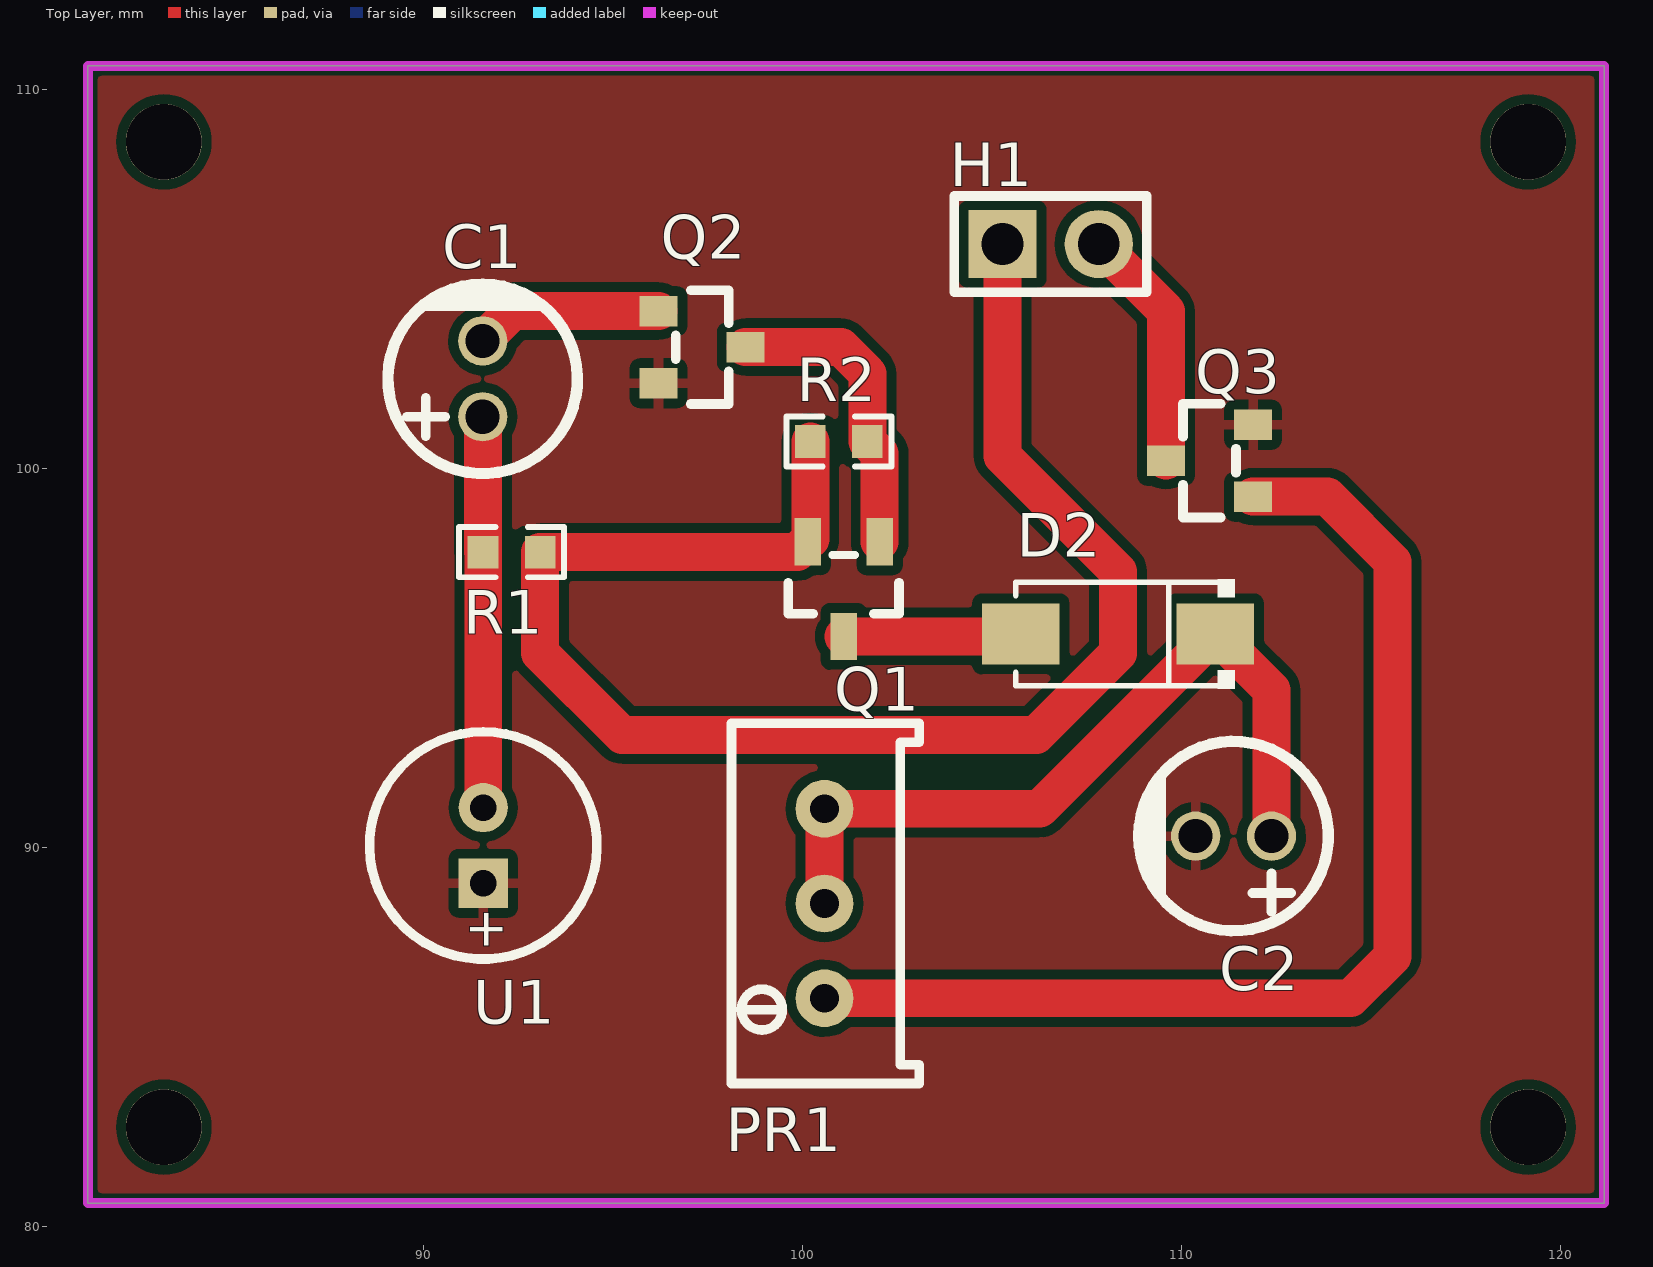
[diagram p0: Top Layer view]
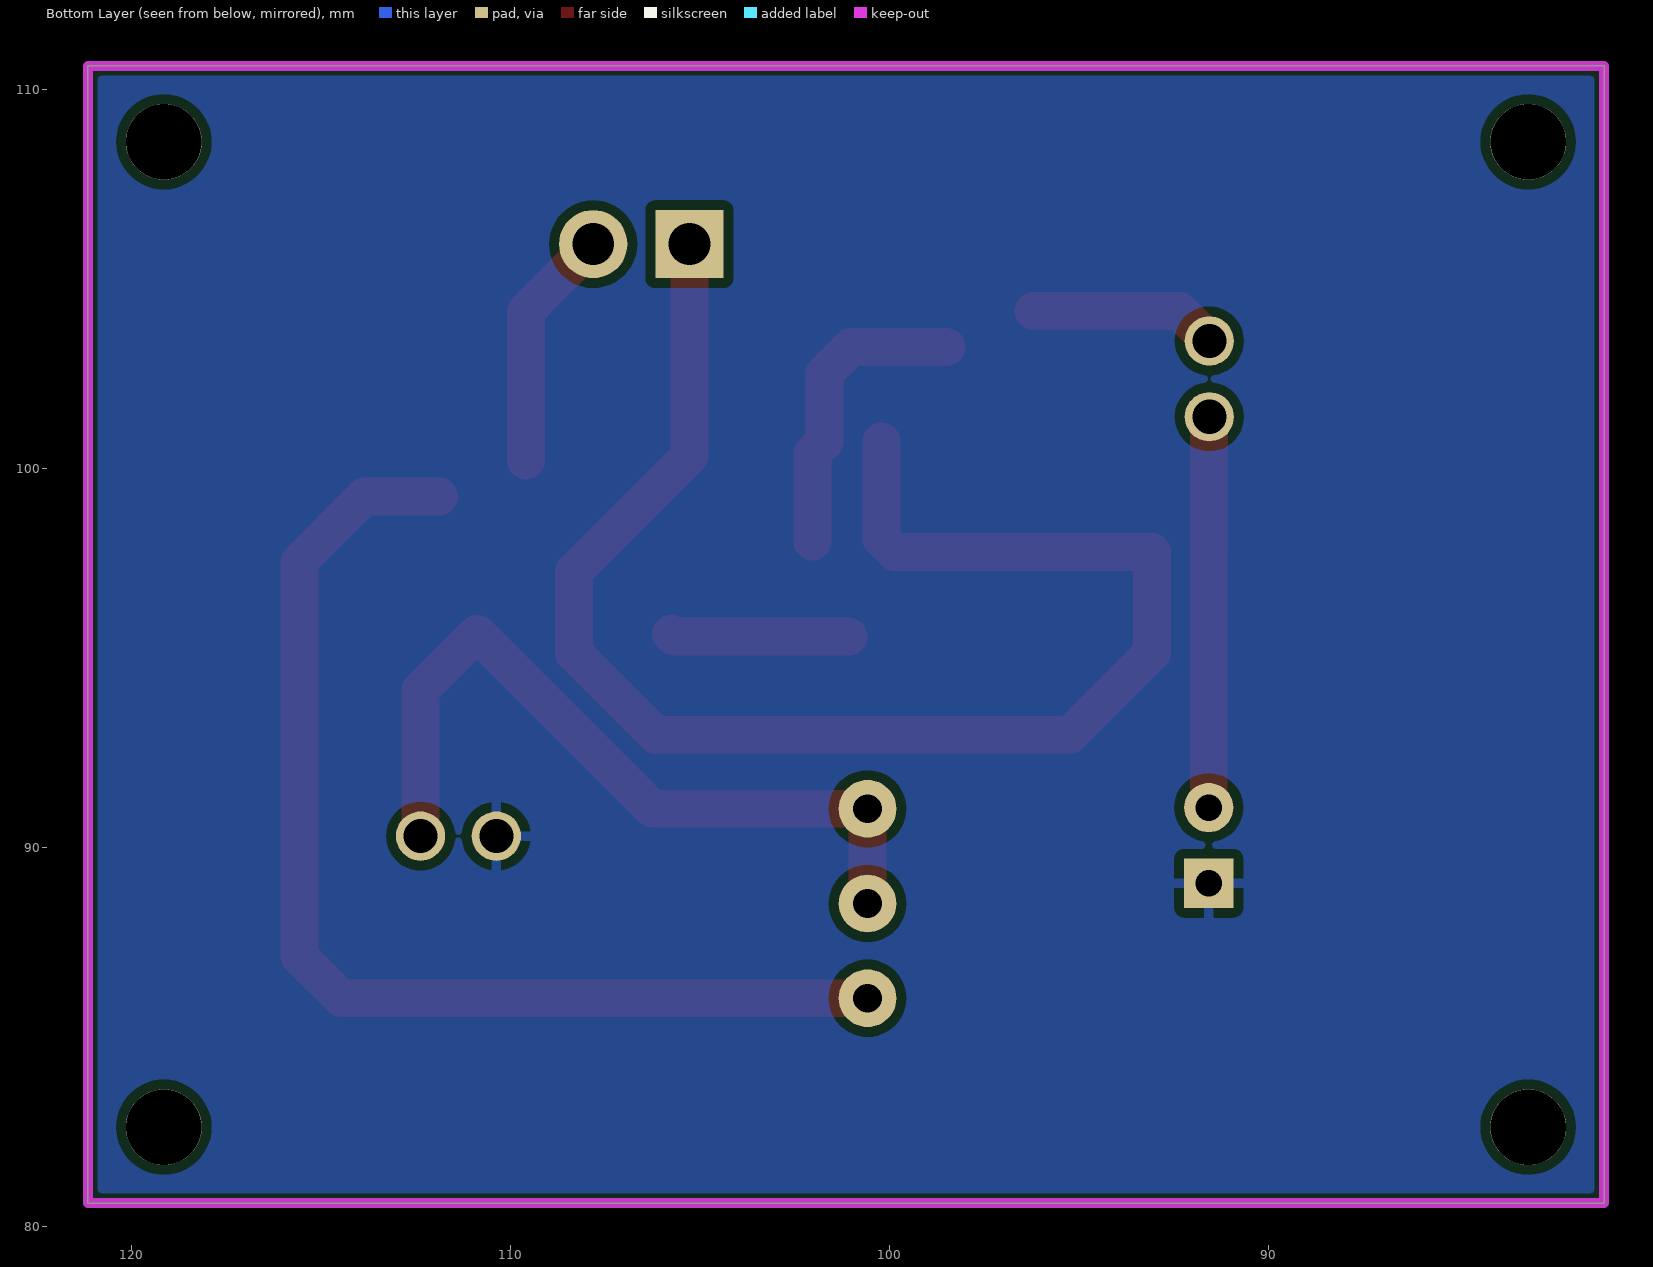
[diagram p1: Bottom Layer view, seen from below]
# Altium PCB MISC49923.pcbdoc
Units mm, origin at the board's own origin, x right, y up, seen from the top; angles counter-clockwise.
Board outline 40 x 30 mm, 2 copper layers (Top Layer, Bottom Layer), stack 1.58 mm thick; 11 components, 9 nets, 30 pads, 0 vias.

## Layer stack, top to bottom
Top Solder Mask Layer: solder mask 0.01, Dk 3.3
Top Layer: signal copper 0.035
Dielectric1: surface 1.51, FR4, Dk 4.5
Bottom Layer: signal copper 0.035
Bottom Solder Mask Layer: solder mask 0.01, Dk 3.3

## Board outline
81.153,110.617 81.153,80.617 121.153,80.617 121.153,110.617

## Design rules (kind name [scope] priority, off if disabled: settings)
BoardOutlineClearance copperThickness2oz_1 [All] p2 off: genericclearance=0.203 ignorepadtopadclearanceinfootprint=FALSE except(0: Arc-SplitContinuation Track-SplitContinuation SMDPad-SplitContinuation THPad-SplitContinuation Via-SplitContinuation Fill-SplitContinuation Region-SplitContinuation Poly-SplitContinuation Text-SplitContinuation Hole-SplitContinuation; 0.152: Arc-CutoutEdge SMDPad-CutoutEdge THPad-CutoutEdge Via-CutoutEdge Fill-CutoutEdge Region-CutoutEdge Text-CutoutEdge; 0.176: Hole-OutlineEdge Hole-CutoutEdge; 0.254: Poly-OutlineEdge Poly-CutoutEdge; 0.3: Arc-OutlineEdge Track-OutlineEdge SMDPad-OutlineEdge THPad-OutlineEdge Via-OutlineEdge Fill-OutlineEdge Region-OutlineEdge Text-OutlineEdge Track-CutoutEdge)
BoardOutlineClearance copperThickness1oz_1 [All] p4: genericclearance=0.102 ignorepadtopadclearanceinfootprint=FALSE except(0: Arc-SplitContinuation Track-SplitContinuation SMDPad-SplitContinuation THPad-SplitContinuation Via-SplitContinuation Fill-SplitContinuation Region-SplitContinuation Poly-SplitContinuation Text-SplitContinuation Hole-SplitContinuation; 0.152: SMDPad-CutoutEdge THPad-CutoutEdge Via-CutoutEdge Fill-CutoutEdge Region-CutoutEdge Text-CutoutEdge; 0.176: Hole-OutlineEdge Hole-CutoutEdge; 0.254: Poly-OutlineEdge Poly-CutoutEdge; 0.3: Arc-OutlineEdge Track-OutlineEdge SMDPad-OutlineEdge THPad-OutlineEdge Via-OutlineEdge Fill-OutlineEdge Region-OutlineEdge Text-OutlineEdge Arc-CutoutEdge Track-CutoutEdge)
Clearance copperThickness2oz [All] p1 off: gap=0.203 ignorepadtopadclearanceinfootprint=FALSE except(0.152: SMDPad-Track SMDPad-SMDPad THPad-Track SMDPad-THPad THPad-THPad Track-Via SMDPad-Via THPad-Via Via-Via Fill-Track Region-Track Fill-SMDPad Region-SMDPad Fill-THPad Region-THPad Fill-Via Region-Via Fill-Fill Fill-Region Region-Region Arc-Track Arc-SMDPad Arc-THPad Arc-Via Fill-Arc Region-Arc Arc-Arc Text-Track SMDPad-Text Text-THPad Text-Via Fill-Text Region-Text Arc-Text Text-Text; 0.176: Hole-Track Hole-SMDPad Hole-THPad Hole-Via Fill-Hole Region-Hole Hole-Arc Hole-Text; 0.254: Poly-Track Poly-SMDPad Poly-THPad Poly-Via Poly-Fill Poly-Region Poly-Poly Poly-Arc Poly-Text Poly-Hole)
Clearance copperThickness1oz [All] p3: gap=0.102 ignorepadtopadclearanceinfootprint=FALSE except(0.152: SMDPad-Track SMDPad-SMDPad THPad-Track SMDPad-THPad THPad-THPad Track-Via SMDPad-Via THPad-Via Via-Via Fill-Track Region-Track Fill-SMDPad Region-SMDPad Fill-THPad Region-THPad Fill-Via Region-Via Fill-Fill Fill-Region Region-Region Arc-Track Arc-SMDPad Arc-THPad Arc-Via Fill-Arc Region-Arc Arc-Arc Text-Track SMDPad-Text Text-THPad Text-Via Fill-Text Region-Text Arc-Text Text-Text; 0.176: Hole-Track Hole-SMDPad Hole-THPad Hole-Via Fill-Hole Region-Hole Hole-Arc Hole-Text; 0.254: Poly-Track Poly-SMDPad Poly-THPad Poly-Via Poly-Fill Poly-Region Poly-Poly Poly-Arc Poly-Text Poly-Hole)
Creepage creepage [All] p1: checkdistance=0 ignoreinternallayers=TRUE applytopolygonpour=TRUE
DiffPairsRouting differentialPair [All] p1: maxlimit=0.152 minlimit=0.152 mostfreqgap=0.152 toplayer_minwidth=0.127 toplayer_prefwidth=0.254 toplayer_maxwidth=2.54 toplayer_mingap=0.152 toplayer_prefgap=0.152 toplayer_maxgap=0.152 bottomlayer_minwidth=0.127 bottomlayer_prefwidth=0.254 bottomlayer_maxwidth=2.54 bottomlayer_mingap=0.152 bottomlayer_prefgap=0.152 bottomlayer_maxgap=0.152 maxuncoupledlength=0.254
HoleToHoleClearance otherClearance [All] p1: gap=0.3 allowstackedmicrovias=TRUE
Length netLength [All] p1: minlimit=0 maxlimit=0
MatchedLengths netLengthTolerance [All] p1: tolerance=25.4
PasteMaskExpansion pasteMaskExpansion [All] p1: expansion=0
PlaneConnect innerPlane [All] p1: planeconnectstyle=Relief reliefexpansion=0.508 reliefentries=4 reliefconductorwidth=0.254 reliefairgap=0.254
PolygonConnect copperRegion [(InNet('GND'))] p1: connectstyle=Relief reliefconductorwidth=0.254 reliefentries=4 polygonreliefangle="90 Angle" airgapwidth=0.254 via.connectstyle=Relief via.reliefconductorwidth=0.254 via.reliefentries=4 via.polygonreliefangle="90 Angle" via.airgapwidth=0.254
RoutingVias viaSize [All] p1: holewidth=0.305 width=0.61 viastyle="Through Hole" minholewidth=0.3 minwidth=0.5 maxholewidth=6.3 maxwidth=10
SolderMaskExpansion solderMaskExpansion [IsVia] p1: expansion=-25.4 istentingtop=TRUE
SolderMaskExpansion solderMaskExpansion [All] p2: expansion=0.051 istentingtop=FALSE
Width copperThickness2oz_2 [All] p1 off: maxlimit=2.54 minlimit=0.203 preferedwidth=0.254
Width copperThickness1oz_2 [All] p2: maxlimit=2.54 minlimit=0.127 preferedwidth=0.254

## Components (designator, comment, footprint, x,y, rotation, side; value= is the part's Value field where it differs from the comment)
C1 "1uF" CAP-TH_BD5.0-P2.00-D0.8-FD-10UF50VC110GL 91.567,102.362 r90 top
C2 "16v" CAP-TH_BD5.0-P2.00-D0.8-FD-10UF50VC110GL 111.379,90.297 r180 top
D2 "" SMA_1N4007 108.331,95.631 r180 top
H1 "" HDR-TH_2P-P2.54-V-M-1 106.553,105.918 r0 top
PR1 "10kΩ" R_3296 100.457,88.519 r90 top
Q1 "" S8550P_SOT 101.092,96.774 r90 top
Q2 "" S8050_SOT-23 97.356,103.198 r180 top
Q3 "" S8050_SOT-23 110.744,100.203 r0 top
R1 "10K" R0603 92.329,97.79 r0 top
R2 "10K" R0603 100.965,100.711 r180 top
U1 "Current source" 咪头 91.582,90.051 r90 top

## Footprints (in the part's own frame and the unit in brackets; to place one, negate y for a bottom-side part, rotate by r counter-clockwise, add the part's x,y. Pads: shape width x height; smd on the part's side, far side on the other; paste and mask are expansions set on the pad)
CAP-TH_BD5.0-P2.00-D0.8-FD-10UF50VC110GL [mm]
  round 1.3 hole 0.9 paste+0 mask+0.051: 1(-1,0) 2(1,0)
  silkscreen extent -2.5,-2.5 2.5,2.5
HDR-TH_2P-P2.54-V-M-1 [mm]
  rect 1.8x1.8 hole 1.1: 1(-1.27,0)
  round 1.8 hole 1.1: 2(1.27,0)
  silkscreen extent -2.54,-1.27 2.54,1.27
R0603 [mm]
  rect 0.806x0.864 smd paste-100 mask+0.051: 1(-0.753,0) 2(0.753,0)
  silkscreen extent -1.39,-0.66 1.39,0.66
R_3296 [mil]
  round 60 hole 30 paste+0 mask+2: 1(-98.4,-5) 2(0,-5) 3(98.4,-5)
  silkscreen extent -187,-103 187,92
S8050_SOT-23 [mm]
  rect 1x0.8 smd paste+0 mask+0.051: 1(1.15,-0.95) 2(1.15,0.95) 3(-1.15,0)
  silkscreen extent -0.7,-1.5 0.7,1.5
S8550P_SOT [mm]
  rect 1.25x0.701 smd paste+0 mask+0.051: 1(1.291,-0.95) 2(1.291,0.95) 3(-1.208,0)
  silkscreen extent -0.61,-1.46 0.94,1.46
SMA_1N4007 [mm]
  rect 2.046x1.62 smd paste+0 mask+0.051: 1(-2.565,0) 2(2.565,0)
  silkscreen extent -3.08,-1.44 2.7,1.44
咪头 [mm]
  rect 1.3x1.3 hole 0.7: 1(-1,0)
  round 1.3 hole 0.7: 2(1,0)
  silkscreen extent -3,-3 3,3

## Free pads (board coordinates)
  round 2 hole 2: 1(83.153,82.617) 1(83.153,108.617) 1(119.153,82.617) 1(119.153,108.617)

## Nets (pads, with @x,y where several pads share a name; then routed paths per layer and width w, separated by ;. In a path a pad name is that pad's centre, name@x,y a point inside that pad or via, vN(x,y) a via of type N, cw(c..) or ccw(c..) an arc to the next point about the centre after c; other vN are vias at no path point)
$1N6: H1.1 Q1.2 R1.2 R2.2 | length 41.6
  Top Layer w1: R2.2 100.212,98.135 Q1.2 99.867,97.79 R1.2 93.082,95.132 95.25,92.964 106.172,92.964 108.331,95.123 108.331,97.282 105.283,100.33 H1.1
$1N7: Q1.1 Q2.3 R2.1 | length 8.1
  Top Layer w1: Q2.3 101.018,103.198 101.718,102.498 R2.1 102.042,100.387 Q1.1
$1N8: D2.2 Q1.3 | length 4.7
  Top Layer w1: Q1.3 105.701,95.566 D2.2
$1N9: C1.2 Q2.1 | length 5
  Top Layer w1: C1.2 92.353,104.148 Q2.1
$1N10: C1.1 R1.1 U1.2 | length 10.3
  Top Layer w1: C1.1 91.576,101.353 R1.1 91.582,97.784 U1.2
$1N12: C2.1 D2.1 PR1.2 PR1.3 | length 20.7
  Top Layer w1: PR1.2 PR1.3 106.258,91.018 110.871,95.631 D2.1 112.379,94.148 C2.1
$1N13: PR1.1 Q3.1 | length 30.2
  Top Layer w1: PR1.1 114.468,86.02 115.57,87.122 115.57,97.536 113.853,99.253 Q3.1
$1N14: H1.2 Q3.3 | length 6.4
  Top Layer w1: H1.2 109.594,104.147 Q3.3
GND: C2.2 Q2.2 Q3.2 U1.1

## Polygon pours and split planes (outlines as drawn)
GND on Top Layer (solid, remove dead copper, pour order 0): 77.597,113.157 77.597,76.2 126.238,76.2 126.238,113.157
GND on Bottom Layer (solid, remove dead copper, pour order 2): 76.2,112.649 76.2,76.327 126.365,76.327 126.365,112.649

## Keep-outs
Board Outline Layer:
  the board outline again, w0.254